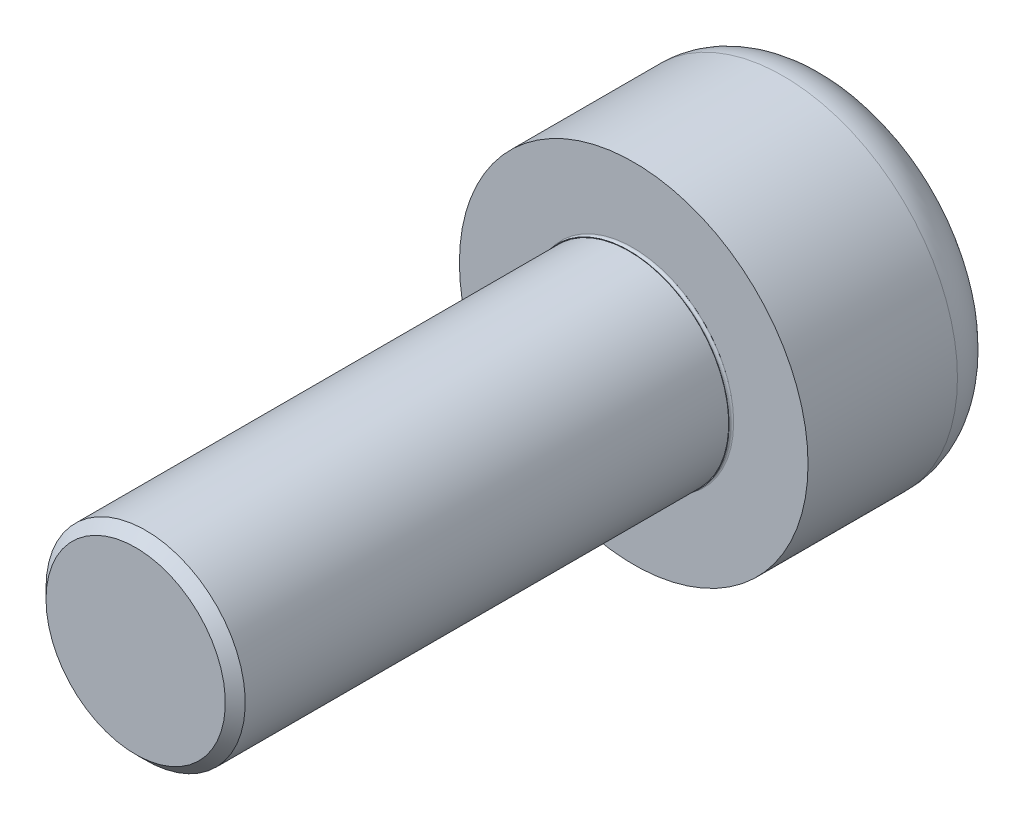
SolidWorks part; units mm, degrees
material "8.8级"
ref_plane "Front" through (0, 0, 0) normal (0, 0, 1) x (1, 0, 0)
ref_plane "Top" through (0, 0, 0) normal (0, 1, 0) x (1, 0, 0)
ref_plane "Right" through (0, 0, 0) normal (1, 0, 0) x (0, 0, -1)
sketch "Logo3_Revol_Axis" plane through (0, 0, 0) normal (0, 1, 0) x (1, 0, 0)
  line L0 (0, -43.5172) -> (0, 43.5172) construction
sketch "Logo3_bib1" plane through (0, 0, 0) normal (0, -1, 0) x (-1, 0, 0)
  line L0 (0, -5) -> (0, 2)
  line L1 (0, 2) -> (1.25, 2)
  line L2 (1.75, 1.5) -> (1.75, 0)
  line L3 (1.75, 0) -> (1, 0)
  line L4 (1, 0) -> (1, -0.01)
  line L5 (1, -4.9) -> (0.9, -5)
  line L6 (0.9, -5) -> (0, -5)
  line L7 (1, -0.01) -> (1.0134, -0.01)
  line L8 (1.0066, -0.0488) -> (1, -0.0464)
  line L9 (1, -0.0464) -> (1, -4.9)
  line L10 (0, 10.5852) -> (0, -63.2873) construction
  arc A0 (1.25, 2) -> (1.75, 1.5) centre (1.25, 1.5) cw
  arc A1 (1.0134, -0.01) -> (1.0066, -0.0488) centre (1.0134, -0.03) ccw
  point P17 (0.9, -0.01)
revolve "Revolve1" add sketch "Logo3_bib1" angle 360 about L10
sketch "Logo3_bib2" plane through (0, 0, -2) normal (0, 0, -1) x (1, 0, 0)
  line L1 (0.866, 0) -> (0.433, 0.75)
  line L2 (0.433, 0.75) -> (-0.433, 0.75)
  line L3 (-0.433, 0.75) -> (-0.866, 0)
  line L4 (-0.866, 0) -> (-0.433, -0.75)
  line L5 (-0.433, -0.75) -> (0.433, -0.75)
  line L6 (0.433, -0.75) -> (0.866, 0)
  circle A0 centre (0, 0) radius 0.75 construction
extrude "Cut-Extrude1" cut sketch "Logo3_bib2" against normal blind 0.75
equation "\"DIA2@XZQB7_bib1\" = \"XZQB7_d1-pas@XZQB7_bib1\""
equation "\"LGT1@XZQB7_bib1\" = \"XZQB7_d1@XZQB7_bib1\""
equation "\"D1@Cut-Extrude1\" = \"XZQB7_c1@XZQB7_bib2\"/2."
